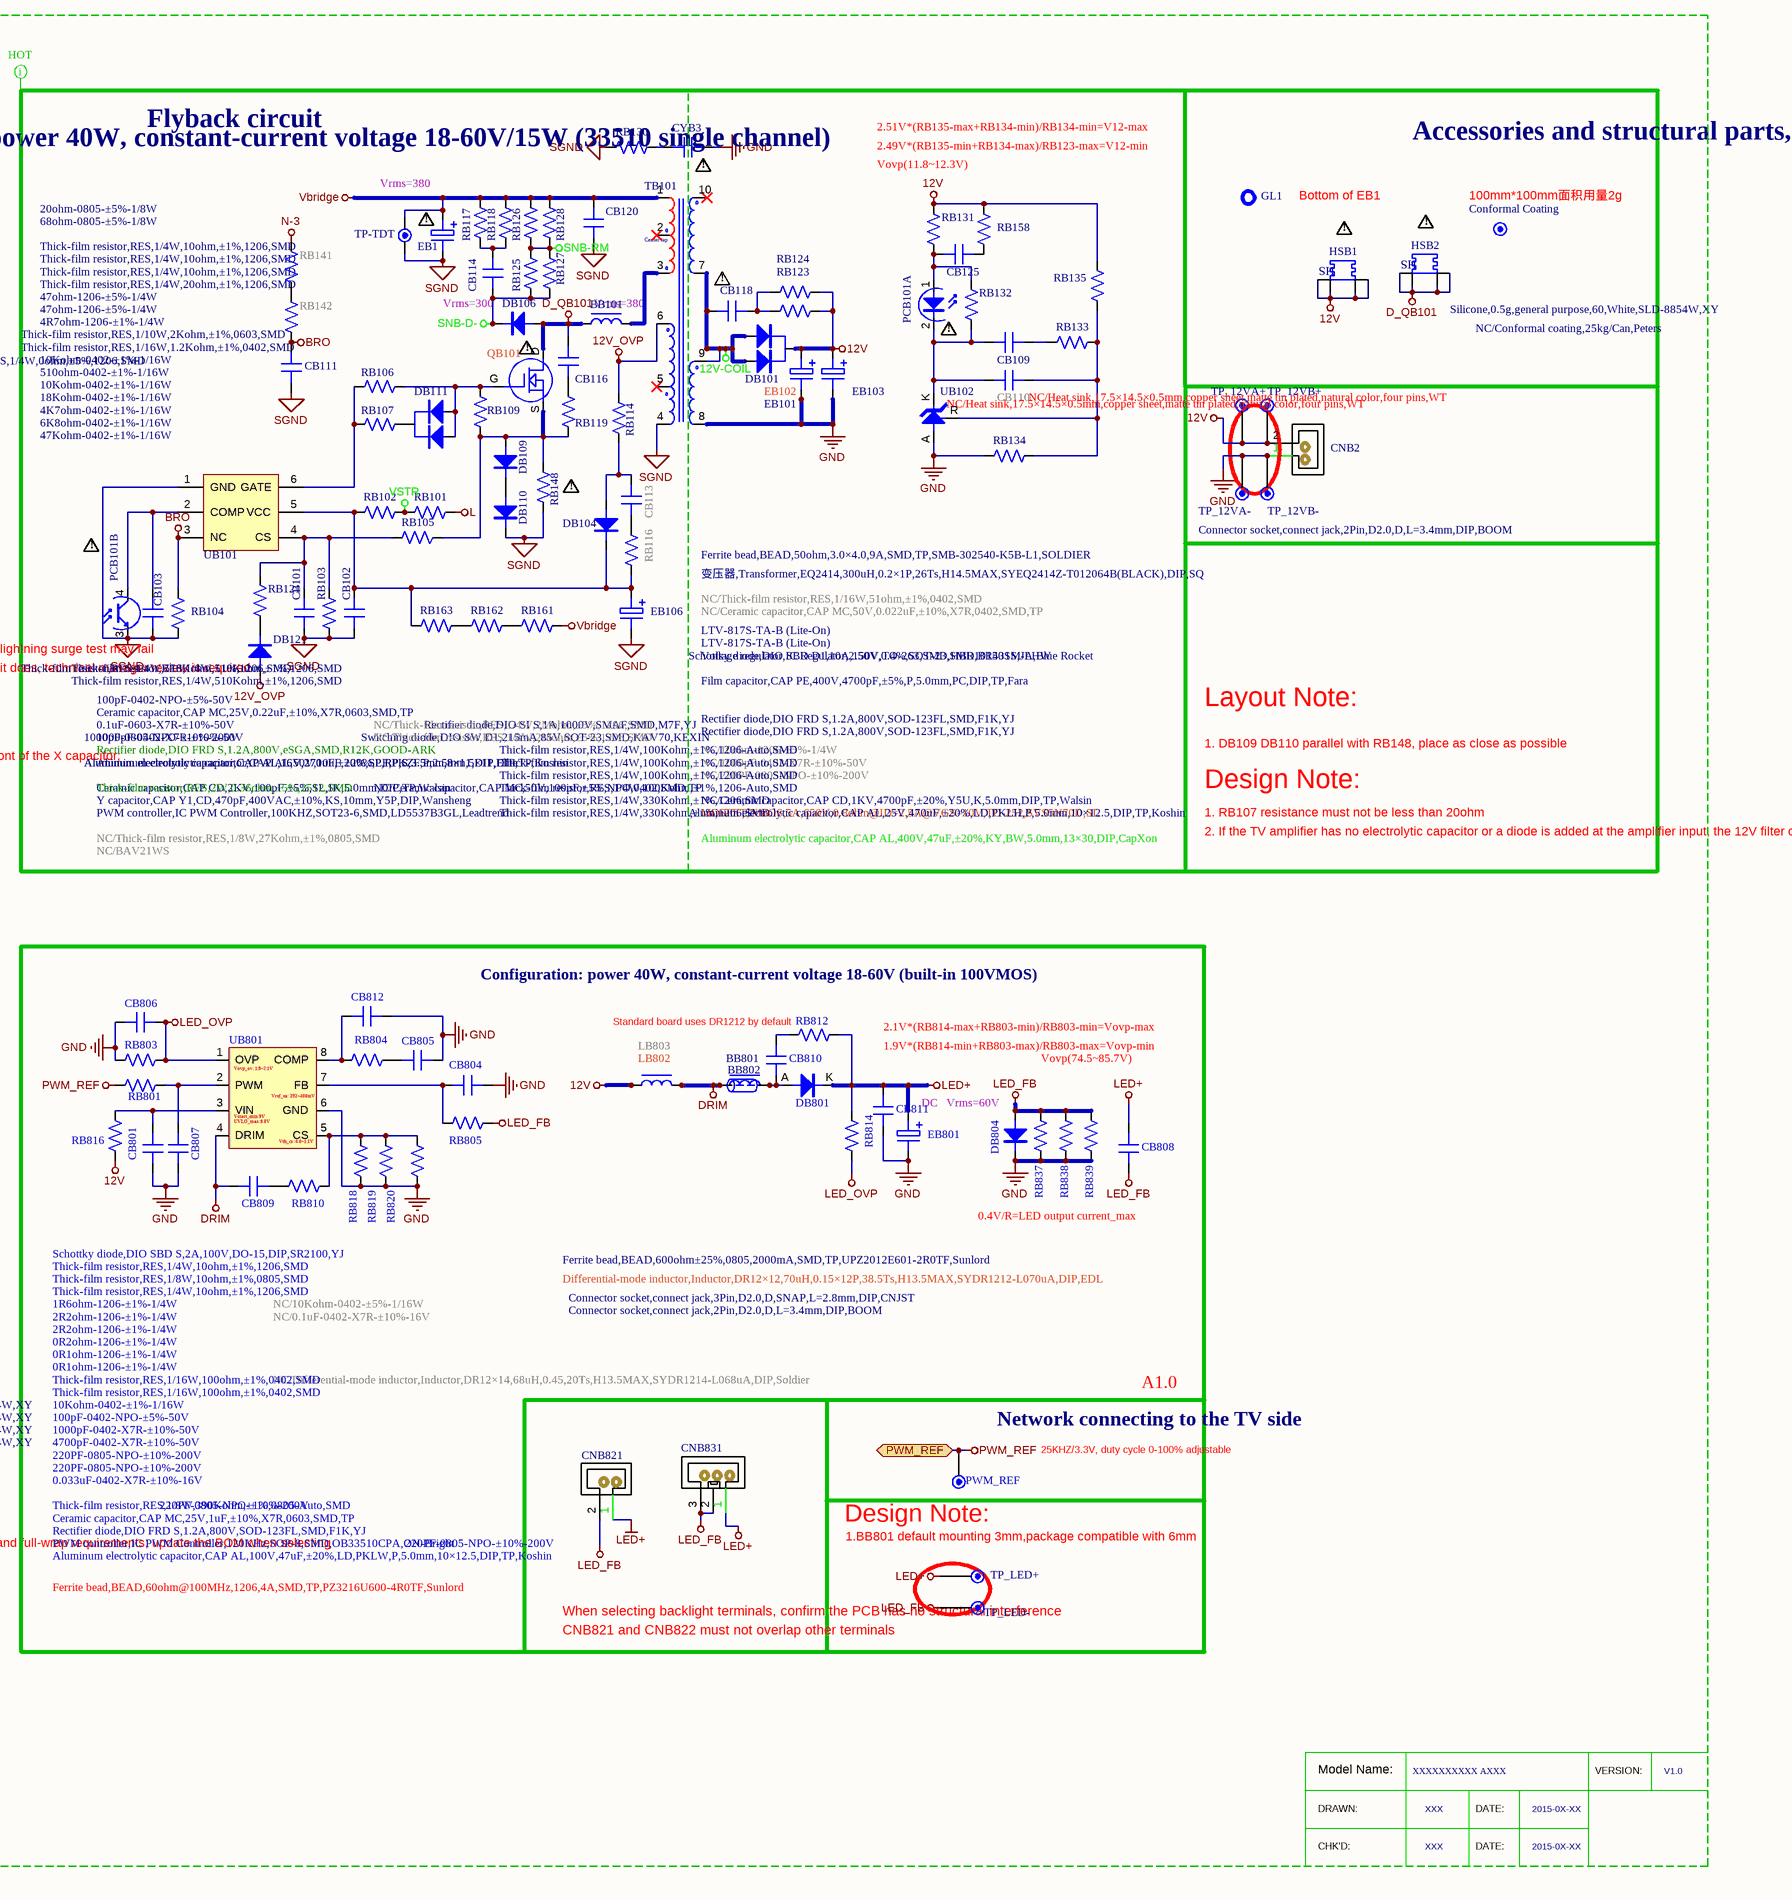
[diagram p0: MISC116569-4.SchDoc, right]
# Altium project MISC116569-15.PrjPCB (part 8 of 8)

## Nets that join several sheets
3V3_STB: MISC116569-6 (7 pins), MISC116569-7 (22 pins), MISC116569-8 (CK1.2 RK4.2 RK13.2), MISC116569-10 (RA35.2), MISC116569-13 (RT1.1)
3V3_Tun: MISC116569-7 (CI18.2 RF43.1 RF44.1), MISC116569-13 (15 pins)
5V_M: MISC116569-6 (7 pins), MISC116569-8 (RK10.2), MISC116569-10 (FU1.2 RO2.1 RU4.2)
5V_STB: MISC116569-6 (19 pins), MISC116569-7 (RF8.2 RF9.2), MISC116569-8 (RK12.2 RK18.2), MISC116569-9 (R5V.1), MISC116569-11 (RPV7.3)
12V: MISC116569-6 (5 pins), MISC116569-9 (R12V.1), MISC116569-12 (12 pins), MISC116569-4 (19 pins)
+1.8V_DDR: MISC116569-6 (5 pins), MISC116569-7 (6 pins)
GND: MISC116569-3 (18 pins), MISC116569-6 (33 pins), MISC116569-7 (40 pins), MISC116569-8 (17 pins), MISC116569-9 (17 pins), MISC116569-10 (59 pins), MISC116569-11 (21 pins), MISC116569-12 (25 pins), MISC116569-13 (53 pins), MISC116569-4 (29 pins)
PWM_REF: MISC116569-6 (CG201.1 RG61.2 RG61.3), MISC116569-4 (PWM_REF.1 RB801.1)
VDDC_CORE: MISC116569-6 (8 pins), MISC116569-7 (13 pins)
AMP_L_OUT_IC: MISC116569-7 (CF29.1 U1.41), MISC116569-10 (CA32.2), MISC116569-12 (RA3.1)
AMP_MUTE_OUT_IC: MISC116569-7 (U1.90), MISC116569-12 (RA1.1 RA2.2)
AMP_R_OUT_IC: MISC116569-7 (CF30.1 U1.42), MISC116569-10 (CA31.2), MISC116569-12 (RA14.1)
AV1_CVBS_IN_IC: MISC116569-7 (U1.31), MISC116569-10 (CI1.1)
AV1_L_IN_IC: MISC116569-7 (U1.37), MISC116569-10 (CI5.1)
AV1_R_IN_IC: MISC116569-7 (U1.38), MISC116569-10 (CI6.1)
CVBS_OUT_IC: MISC116569-7 (U1.33), MISC116569-10 (CO18.2 RO17.1 RO18.2)
EPH_DET_IN_IC: MISC116569-7 (U1.58), MISC116569-10 (CA33.2 RA36.1)
HDMI_A_0N_IN_IC: MISC116569-7 (U1.1), MISC116569-11 (JH1.9)
HDMI_A_0P_IN_IC: MISC116569-7 (U1.2), MISC116569-11 (JH1.7)
HDMI_A_1N_IN_IC: MISC116569-7 (U1.3), MISC116569-11 (JH1.6)
HDMI_A_1P_IN_IC: MISC116569-7 (U1.4), MISC116569-11 (JH1.4)
HDMI_A_2N_IN_IC: MISC116569-7 (U1.5), MISC116569-11 (JH1.3)
HDMI_A_2P_IN_IC: MISC116569-7 (U1.6), MISC116569-11 (JH1.1)
HDMI_A_CKN_IN_IC: MISC116569-7 (U1.127), MISC116569-11 (JH1.12)
HDMI_A_CKP_IN_IC: MISC116569-7 (U1.128), MISC116569-11 (JH1.10)
HDMI_A_HPD_OUT_IC: MISC116569-7 (U1.120), MISC116569-11 (RH4.6 RH4.8)
HDMI_A_SCL_IN_IC: MISC116569-7 (U1.107), MISC116569-11 (RH6.2)
HDMI_A_SDA_IO_IC: MISC116569-7 (U1.106), MISC116569-11 (RH5.2)
HDMI_ARC_OUT_IC: MISC116569-7 (U1.125), MISC116569-11 (CH81.2)
HDMI_CEC_IO_IC: MISC116569-7 (U1.119), MISC116569-11 (RH83.1)
HDMI_DET: MISC116569-7 (U1.110), MISC116569-11 (RH81.1 RH82.1)
IR_IN_IC: MISC116569-7 (U1.97), MISC116569-8 (CK6.2 RK19.2)
KEY_IN_IC: MISC116569-7 (U1.109), MISC116569-8 (CK2.1 RK3.1)
LED_OUT_IC: MISC116569-7 (U1.92), MISC116569-8 (RK13.1 RK14.1 RK15.2)
LINE_L_OUT_IC: MISC116569-7 (U1.39), MISC116569-10 (CO11.2 RO12.1)
LINE_R_OUT_IC: MISC116569-7 (U1.40), MISC116569-10 (CO14.2 RO15.1)
LVDS_E0N_IC: MISC116569-7 (U1.76), MISC116569-9 (CNW1.19 CNW2.19)
LVDS_E0P_IC: MISC116569-7 (U1.75), MISC116569-9 (CNW1.20 CNW2.20)
LVDS_E1N_IC: MISC116569-7 (U1.74), MISC116569-9 (CNW1.21 CNW2.21)
LVDS_E1P_IC: MISC116569-7 (U1.73), MISC116569-9 (CNW1.22 CNW2.22)
LVDS_E2N_IC: MISC116569-7 (U1.72), MISC116569-9 (CNW1.23 CNW2.23)
LVDS_E2P_IC: MISC116569-7 (U1.71), MISC116569-9 (CNW1.24 CNW2.24)
LVDS_E3N_IC: MISC116569-7 (U1.68), MISC116569-9 (CNW1.29 CNW2.29)
LVDS_E3P_IC: MISC116569-7 (U1.67), MISC116569-9 (CNW1.30 CNW2.30)
LVDS_ECKN_IC: MISC116569-7 (U1.70), MISC116569-9 (CNW1.27 CNW2.27)
LVDS_ECKP_IC: MISC116569-7 (U1.69), MISC116569-9 (CNW1.28 CNW2.28)
LVDS_O0N_IC: MISC116569-7 (U1.89), MISC116569-9 (CNW1.7 CNW2.7)
LVDS_O0P_IC: MISC116569-7 (U1.88), MISC116569-9 (CNW1.8 CNW2.8)
LVDS_O1N_IC: MISC116569-7 (U1.87), MISC116569-9 (CNW1.9 CNW2.9)
LVDS_O1P_IC: MISC116569-7 (U1.86), MISC116569-9 (CNW1.10 CNW2.10)
LVDS_O2N_IC: MISC116569-7 (U1.84), MISC116569-9 (CNW1.11 CNW2.11)
LVDS_O2P_IC: MISC116569-7 (U1.83), MISC116569-9 (CNW1.12 CNW2.12)
LVDS_O3N_IC: MISC116569-7 (U1.80), MISC116569-9 (CNW1.17 CNW2.17)
LVDS_O3P_IC: MISC116569-7 (U1.79), MISC116569-9 (CNW1.18 CNW2.18)
LVDS_OCKN_IC: MISC116569-7 (U1.82), MISC116569-9 (CNW1.15 CNW2.15)
LVDS_OCKP_IC: MISC116569-7 (U1.81), MISC116569-9 (CNW1.16 CNW2.16)
MAIN_SCL_OUT_IC: MISC116569-7 (DI11.K RF43.2 U1.52), MISC116569-13 (RT15.2)
MAIN_SDA_IO_IC: MISC116569-7 (DI10.K RF44.2 U1.51), MISC116569-13 (RT14.2)
PANEL_EN_OUT_IC: MISC116569-7 (U1.93), MISC116569-9 (RM11.1)
POWER_EN_OUT_IC: MISC116569-6 (RM1.1 RM2.1), MISC116569-7 (U1.57)
PWM1: MISC116569-6 (RG61.1), MISC116569-7 (RF13.1 U1.96)
SPDIF_OUT_IC: MISC116569-7 (U1.94), MISC116569-10 (CO31.2 RO21.2)
TUNER_IF_N_IN_IC: MISC116569-7 (U1.45), MISC116569-13 (CT15.2)
TUNER_IF_P_IN_IC: MISC116569-7 (U1.44), MISC116569-13 (CT16.1)
UART_RX_IC: MISC116569-7 (D102.K RF9.1 U1.104), MISC116569-11 (RH89.2)
UART_TX_IC: MISC116569-7 (D101.K RF8.1 U1.103), MISC116569-11 (RH88.1)
USB0_DM_IO_IC: MISC116569-7 (U1.63), MISC116569-10 (DU3.K RU3.1)
USB0_DP_IO_IC: MISC116569-7 (U1.64), MISC116569-10 (DU4.K RU5.1)
XTAL_OUT: MISC116569-7 (L6.2 L6.3), MISC116569-13 (CT11.2 UT1.17)
YPP_Pb&B_IN_IC: MISC116569-7 (U1.26), MISC116569-10 (CV3.2)
YPP_Pr&R_IN_IC: MISC116569-7 (U1.29), MISC116569-10 (CV1.2)
YPP_Y&G_IN_IC: MISC116569-7 (U1.27), MISC116569-10 (CV2.2)